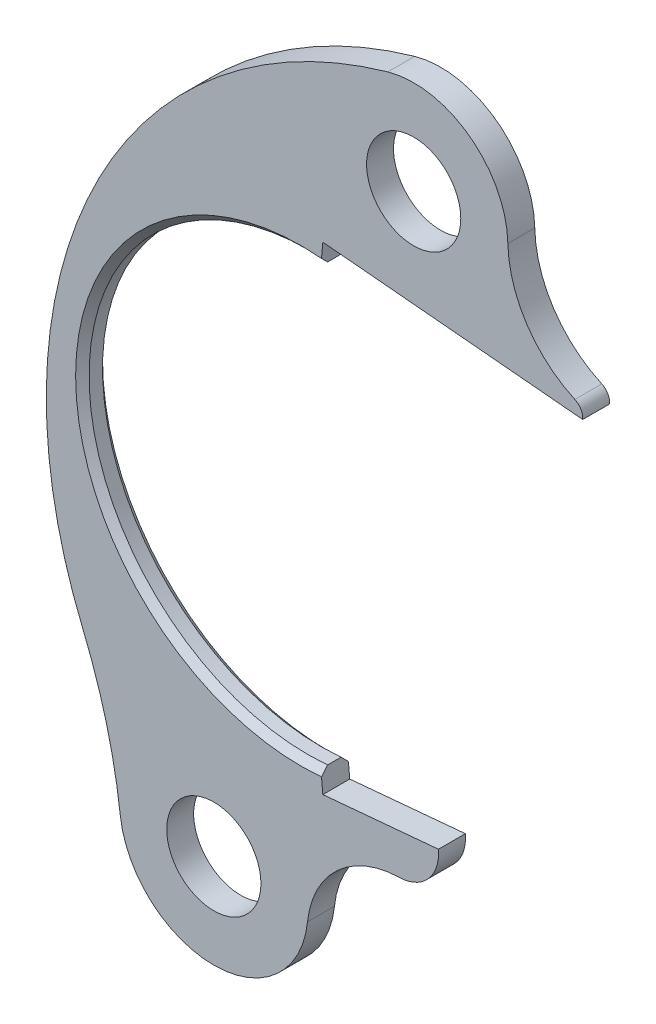
from build123d import *

# Parameters (mm, degrees)
SKETCH1_R           = 35
BOSS_EXTRUDE1_DEPTH = 20
CHAMFER1_SIZE       = 5


with BuildPart() as part:
    # Sketch1 → Boss-Extrude1 (new body)
    with BuildSketch(Plane.XY):
        with BuildLine():
            ThreePointArc((72.887397787, -202.60557658), (27.017010086, -221.097976732), (4.818924287, -265.294201888))
            ThreePointArc((4.818924287, -265.294201888), (-64.294796067, -327.998176898), (-134.306386999, -266.298323103))
            ThreePointArc((-134.306386999, -266.298323103), (-144.622358434, -212.04763629), (-162.31184025, -159.734745723))
            ThreePointArc((-162.31184025, -159.734745723), (-154.669991707, 126.763312998), (64.446169212, 311.5))
            ThreePointArc((64.446169212, 311.5), (125.230637191, 300.548967821), (153.683278213, 245.729957687))
            ThreePointArc((153.683278213, 245.729957687), (167.70153078, 200.795951222), (203.480405215, 170.210848864))
            ThreePointArc((203.480405215, 170.210848864), (207.986601411, 166.133457037), (209.3, 160.2))
            Line((209.3, 160.2), (16.2, 177.8))
            Line((16.2, 177.8), (14.744884523, 161.829658531))
            ThreePointArc((14.744884523, 161.829658531), (-162.499999947, -0.00413168), (14.753113776, -161.828908523))
            Line((14.753113776, -161.828908523), (16.2, -177.7))
            Line((16.2, -177.7), (102.1, -169.9))
            ThreePointArc((102.1, -169.9), (94.597243609, -192.597670349), (72.887397787, -202.60557658))
        make_face()
        with Locations((-64.8, -258)):
            Circle(SKETCH1_R, mode=Mode.SUBTRACT)
        with Locations((83.7, 244.2)):
            Circle(SKETCH1_R, mode=Mode.SUBTRACT)
    extrude(amount=BOSS_EXTRUDE1_DEPTH)

    # Chamfer1
    chamfer1_edges = [part.edges().sort_by_distance(p)[0] for p in [
        (-162.499999947, -0.00413168, 0),
        (-162.499999947, -0.00413168, 20),
    ]]
    chamfer(chamfer1_edges, length=CHAMFER1_SIZE)


solid = part.part
